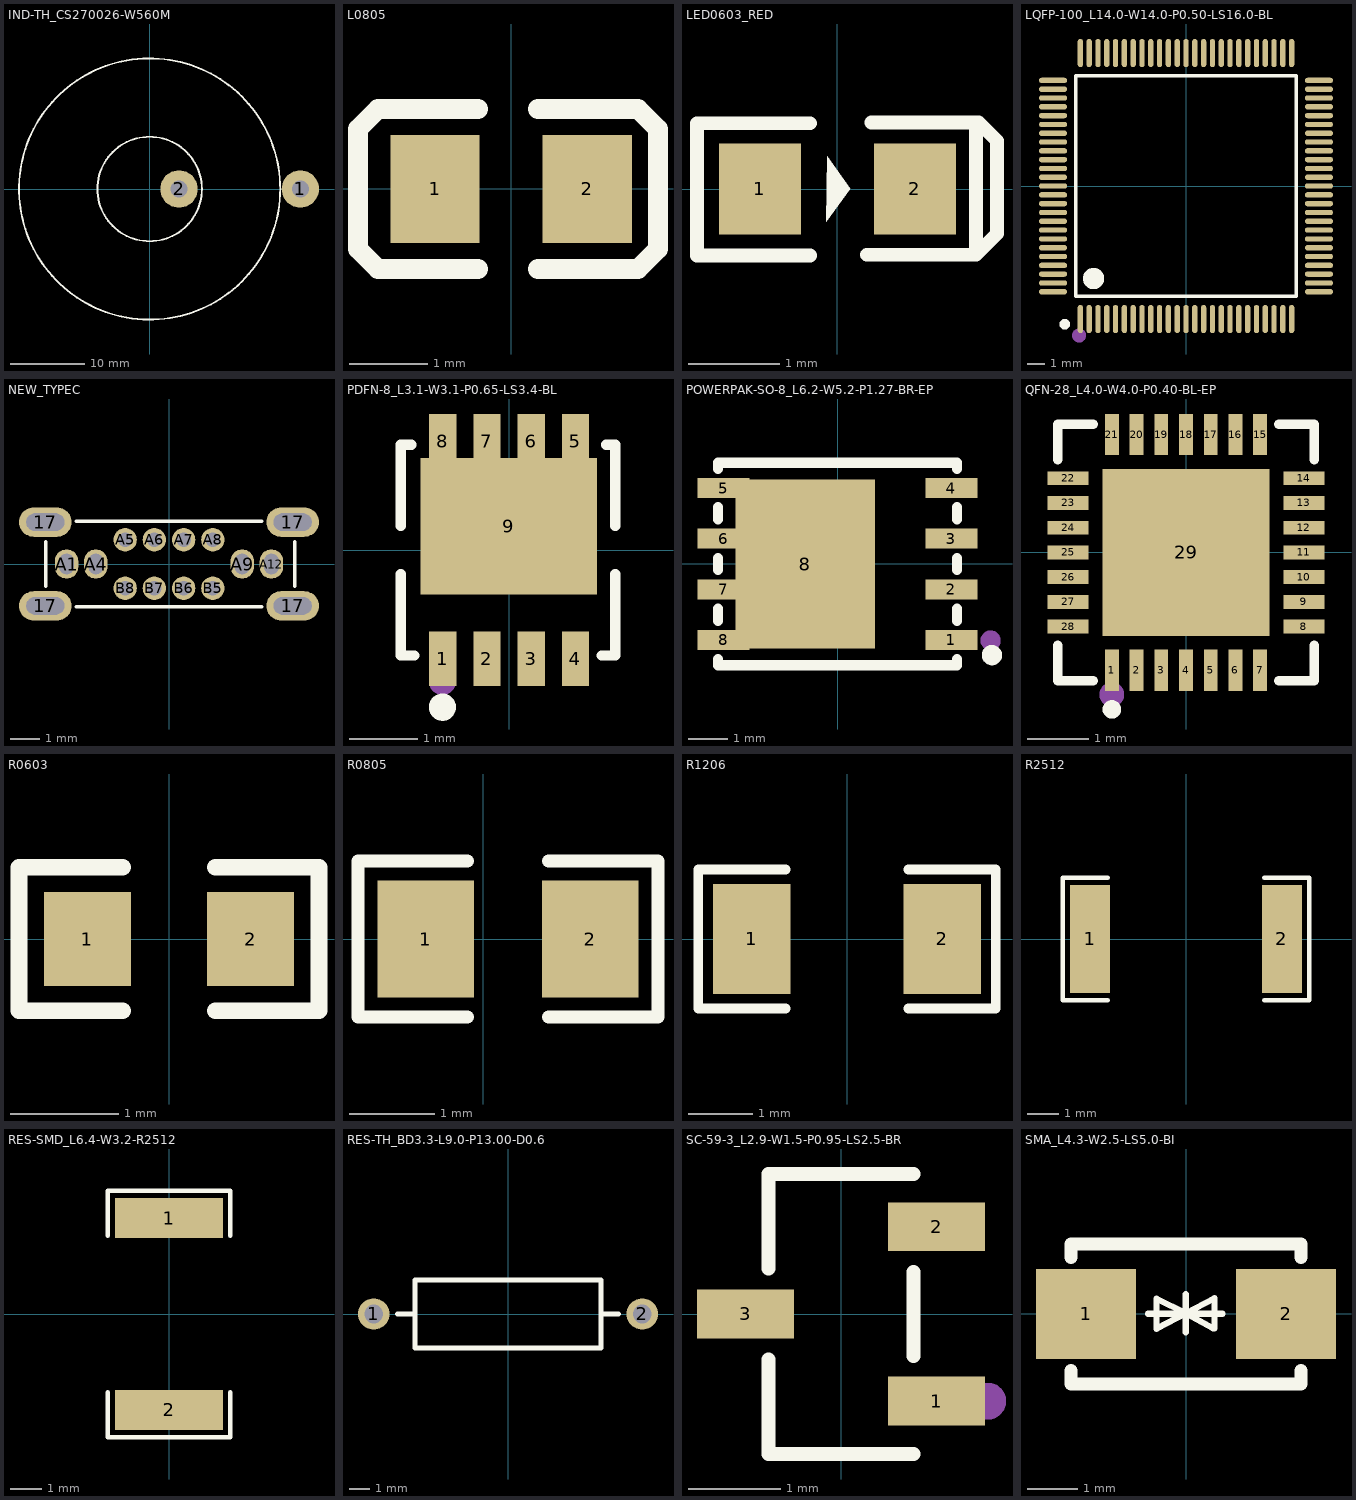
[diagram p0: the footprints below, top view; thin cyan lines are the x and y axes]
# Altium footprint library MISC84402-2.PcbLib: 69 footprints (part 3 of 5)
Each footprint in its own frame and in the unit in brackets; x right, y up, seen from the top. Pads: shape width x height; smd on the part's side, far side on the other; paste and mask are expansions set on the pad; w line width, h text height; cw(c..) or ccw(c..) is an arc to the next point about the centre after c.

## IND-TH_CS270026-W560M [mm]
pads (2):
  round 5 hole 2.3: 1(20.193,0) 2(3.937,0)
Top Overlay:
  circle w0.254: c0,0 r17.5
  circle w0.254: c0,0 r7

## L0805 [mm]
pads (2):
  rect 1.133x1.377 smd: 1(-0.966,0) 2(0.966,0)
Top Overlay:
  lines w0.254: -0.421,-1.016 -1.691,-1.016 -1.945,-0.762 -1.945,-0.635 -1.945,0.762 -1.691,1.016 -1.564,1.016 -0.421,1.016 ; 0.341,-1.016 1.484,-1.016 1.611,-1.016 1.865,-0.762 1.865,0.635 1.865,0.762 1.611,1.016 0.341,1.016
Top Paste:
  region: -0.36,-0.22 -0.36,0.22 -0.745,0.688 -1.433,0.688 -1.533,0.588 -1.533,-0.589 -1.433,-0.689 -0.745,-0.689
  region: 0.36,-0.22 0.36,0.22 0.745,0.688 1.433,0.688 1.533,0.588 1.533,-0.589 1.433,-0.689 0.745,-0.689

## LED0603_RED [mm]
pads (2):
  rect 0.9x1 smd: 1(-0.85,0) 2(0.85,0)
Top Overlay:
  region: -0.11,0.36 -0.12,-0.36 0.14,0
  lines w0.15: -0.3,-0.73 -1.54,-0.73 -1.54,0.72 -0.3,0.72 ; 0.32,-0.72 1.52,-0.72 ; 0.37,0.73 1.52,0.73 ; 1.52,-0.72 1.52,0.73 ; 1.52,-0.72 1.72,-0.52 1.75,-0.49 1.75,0.53 1.55,0.73 1.52,0.73

## LQFP-100_L14.0-W14.0-P0.50-LS16.0-BL [mm]
pads (100):
  oval 0.3x1.6 smd: 1(-6,-7.55) 2(-5.5,-7.55) 3(-5,-7.55) 4(-4.5,-7.55) 5(-4,-7.55) 6(-3.5,-7.55) 7(-3,-7.55) 8(-2.5,-7.55) 9(-2,-7.55) 10(-1.5,-7.55) 11(-1,-7.55) 12(-0.5,-7.55) 13(0,-7.55) 14(0.5,-7.55) 15(1,-7.55) 16(1.5,-7.55) 17(2,-7.55) 18(2.5,-7.55) 19(3,-7.55) 20(3.5,-7.55) 21(4,-7.55) 22(4.5,-7.55) 23(5,-7.55) 24(5.5,-7.55) 25(6,-7.55) 51(6,7.55) 52(5.5,7.55) 53(5,7.55) 54(4.5,7.55) 55(4,7.55) 56(3.5,7.55) 57(3,7.55) 58(2.5,7.55) 59(2,7.55) 60(1.5,7.55) 61(1,7.55) 62(0.5,7.55) 63(0,7.55) 64(-0.5,7.55) 65(-1,7.55) 66(-1.5,7.55) 67(-2,7.55) 68(-2.5,7.55) 69(-3,7.55) 70(-3.5,7.55) 71(-4,7.55) 72(-4.5,7.55) 73(-5,7.55) 74(-5.5,7.55) 75(-6,7.55)
  oval 1.6x0.3 smd: 26(7.55,-6) 27(7.55,-5.5) 28(7.55,-5) 29(7.55,-4.5) 30(7.55,-4) 31(7.55,-3.5) 32(7.55,-3) 33(7.55,-2.5) 34(7.55,-2) 35(7.55,-1.5) 36(7.55,-1) 37(7.55,-0.5) 38(7.55,0) 39(7.55,0.5) 40(7.55,1) 41(7.55,1.5) 42(7.55,2) 43(7.55,2.5) 44(7.55,3) 45(7.55,3.5) 46(7.55,4) 47(7.55,4.5) 48(7.55,5) 49(7.55,5.5) 50(7.55,6) 76(-7.55,6) 77(-7.55,5.5) 78(-7.55,5) 79(-7.55,4.5) 80(-7.55,4) 81(-7.55,3.5) 82(-7.55,3) 83(-7.55,2.5) 84(-7.55,2) 85(-7.55,1.5) 86(-7.55,1) 87(-7.55,0.5) 88(-7.55,0) 89(-7.55,-0.5) 90(-7.55,-1) 91(-7.55,-1.5) 92(-7.55,-2) 93(-7.55,-2.5) 94(-7.55,-3) 95(-7.55,-3.5) 96(-7.55,-4) 97(-7.55,-4.5) 98(-7.55,-5) 99(-7.55,-5.5) 100(-7.55,-6)
Top Overlay:
  lines w0.2: -6.25,-6.25 6.25,-6.25 6.25,6.25 -6.25,6.25 -6.25,-6.25
  lines w0.3: -6.883,-7.696 ccw(c-6.882,-7.846) -6.881,-7.696
  lines w0.6: -5.25,-4.95 ccw(c-5.248,-5.25) -5.245,-4.95
Mechanical 15:
  circle w0.4: c-6.071,-8.484 r0.2

## NEW_TYPEC [mm]
pads (16):
  oval 1.8x1 hole 0.6 slot 1.3 at 0 deg: 17(-4.225,-1.43) 17(-4.225,1.43) 17(4.225,-1.43) 17(4.225,1.43)
  oval 0.8x1 hole 0.5 slot 0.7 at 90 deg: A1(-3.5,0) A4(-2.5,0) A9(2.5,0) A12(3.5,0)
  round 0.8 hole 0.5: A5(-1.5,0.825) A6(-0.5,0.825) A7(0.5,0.825) A8(1.5,0.825) B5(1.5,-0.825) B6(0.5,-0.825) B7(-0.5,-0.825) B8(-1.5,-0.825)
Top Overlay:
  lines w0.127: -4.215,-0.762 -4.215,0.762 ; -3.158,-1.46 3.158,-1.46 ; -3.158,1.461 3.158,1.461 ; 4.294,-0.762 4.294,0.762

## PDFN-8_L3.1-W3.1-P0.65-LS3.4-BL [mm]
pads (9):
  rect 0.4x0.8 smd: 1(-0.975,-1.6) 2(-0.325,-1.6) 3(0.325,-1.6) 4(0.975,-1.6) 5(0.975,1.6) 6(0.325,1.6) 7(-0.325,1.6) 8(-0.975,1.6)
  rect 2.6x2 smd: 9(-0.005,0.35)
Top Overlay:
  circle w0.2: c-0.98,-2.31 r0.1
  lines w0.152: -1.592,-0.354 -1.592,-1.55 -1.396,-1.55 ; -1.592,0.354 -1.592,1.55 -1.434,1.55 ; 1.362,-1.55 1.56,-1.55 1.56,-0.354 ; 1.425,1.55 1.56,1.55 1.56,0.354
Top Paste:
  region: -0.775,1.5 -1.175,1.5 -1.175,2 -0.775,2
  region: 0.775,-2 0.775,-1.2 1.175,-1.2 1.175,-2
  region: 0.125,-2 0.125,-1.2 0.525,-1.2 0.525,-2
  region: -0.525,-2 -0.525,-1.2 -0.125,-1.2 -0.125,-2
  region: -1.175,-2 -1.175,-1.2 -0.775,-1.2 -0.775,-2
  region: -1.31,1.22 1.293,1.22 1.293,-0.649 -1.307,-0.649
  region: -0.125,1.5 -0.525,1.5 -0.525,2 -0.125,2
  region: 0.525,1.5 0.125,1.5 0.125,2 0.525,2
  region: 1.175,1.5 0.775,1.5 0.775,2 1.175,2
Mechanical 15:
  circle w0.2: c-0.98,-1.93 r0.1

## POWERPAK-SO-8_L6.2-W5.2-P1.27-BR-EP [mm]
pads (9):
  rect 1.3x0.5 smd: 1(2.858,-1.905) 2(2.858,-0.635) 3(2.858,0.635) 4(2.858,1.905) 5(-2.858,1.905) 6(-2.858,0.635) 7(-2.858,-0.635) 8(-2.858,-1.905)
  rect 3.5x4.25 smd: 8(-0.813,0)
Top Overlay:
  circle w0.254: c3.873,-2.286 r0.127
  lines w0.254: -3,-2.386 -3,-2.54 3,-2.54 3,-2.386 ; -3,-1.424 -3,-1.116 ; -3,-0.154 -3,0.154 ; -3,1.116 -3,1.424 ; -3,2.386 -3,2.54 3,2.54 3,2.386 ; 3,-1.424 3,-1.116 ; 3,-0.154 3,0.154 ; 3,1.116 3,1.424
Top Paste:
  region: 0.86,1.991 0.86,0.171 -1.94,0.171 -1.94,1.991
  region: -1.94,-1.978 -1.94,-0.158 0.86,-0.158 0.86,-1.978
  region: 2.19,-2.185 2.19,-1.665 3.49,-1.665 3.49,-2.185
  region: 2.19,-0.915 2.19,-0.395 3.49,-0.395 3.49,-0.915
  region: 2.19,0.355 2.19,0.875 3.49,0.875 3.49,0.355
  region: 2.19,1.625 2.19,2.145 3.49,2.145 3.49,1.625
  region: -3.525,-2.185 -3.525,-1.665 -2.225,-1.665 -2.225,-2.185
  region: -3.525,-0.915 -3.525,-0.395 -2.225,-0.395 -2.225,-0.915
  region: -3.525,0.355 -3.525,0.875 -2.225,0.875 -2.225,0.355
  region: -3.525,1.625 -3.525,2.145 -2.225,2.145 -2.225,1.625
Mechanical 15:
  circle w0.254: c3.84,-1.92 r0.127

## QFN-28_L4.0-W4.0-P0.40-BL-EP [mm]
pads (29):
  rect 0.224x0.665 smd: 1(-1.2,-1.907) 2(-0.8,-1.907) 3(-0.4,-1.907) 4(0,-1.907) 5(0.4,-1.907) 6(0.8,-1.907) 7(1.2,-1.907) 15(1.2,1.908) 16(0.8,1.908) 17(0.4,1.908) 18(0,1.908) 19(-0.4,1.908) 20(-0.8,1.908) 21(-1.2,1.908)
  rect 0.665x0.224 smd: 8(1.907,-1.2) 9(1.907,-0.8) 10(1.907,-0.4) 11(1.907,0) 12(1.907,0.4) 13(1.907,0.8) 14(1.907,1.2) 22(-1.907,1.2) 23(-1.907,0.8) 24(-1.907,0.4) 25(-1.907,0) 26(-1.907,-0.4) 27(-1.907,-0.8) 28(-1.907,-1.2)
  rect 2.7x2.7 smd: 29(0,0)
Top Overlay:
  circle w0.15: c-1.2,-2.54 r0.075
  lines w0.152: -2.076,-1.503 -2.076,-2.076 -1.503,-2.076 ; -2.076,1.503 -2.076,2.076 -1.503,2.076 ; 1.503,-2.076 2.076,-2.076 2.076,-1.503 ; 1.503,2.076 2.076,2.076 2.076,1.503
Mechanical 15:
  circle w0.2: c-1.2,-2.3 r0.1

## R0603 [mm]
pads (2):
  rect 0.806x0.864 smd: 1(-0.753,0) 2(0.753,0)
Top Overlay:
  lines w0.152: -0.426,-0.661 -1.385,-0.661 -1.385,0.661 -0.426,0.661 ; 0.426,-0.661 1.385,-0.661 1.385,0.661 0.426,0.661
Top Paste:
  region: -0.355,0.4 -0.355,0.172 -0.735,0.172 -0.735,-0.158 -0.355,-0.158 -0.355,-0.4 -0.405,-0.45 -1.195,-0.45 -1.245,-0.4 -1.245,0.4 -1.195,0.45 -0.405,0.45
  region: 1.195,0.45 0.395,0.45 0.345,0.4 0.345,0.172 0.715,0.172 0.715,-0.158 0.345,-0.158 0.345,-0.4 0.395,-0.45 1.195,-0.45 1.245,-0.4 1.245,0.4

## R0805 [mm]
pads (2):
  rect 1.133x1.377 smd: 1(-0.678,0) 2(1.254,0)
Top Overlay:
  lines w0.152: -0.188,-0.917 -1.473,-0.917 -1.473,0.917 -0.188,0.917 ; 0.764,-0.917 2.049,-0.917 2.049,0.917 0.764,0.917
Top Paste:
  region: -1.412,-0.64 -1.412,0.64 -1.362,0.69 -0.212,0.69 -0.162,0.64 -0.157,0.23 -0.607,0.23 -0.607,-0.22 -0.167,-0.22 -0.162,-0.64 -0.212,-0.69 -1.362,-0.69
  region: 0.738,-0.64 0.738,-0.22 1.183,-0.22 1.183,0.23 0.743,0.23 0.738,0.64 0.788,0.69 1.938,0.69 1.988,0.64 1.988,-0.64 1.938,-0.69 0.788,-0.69

## R1206 [mm]
height 12.5
pads (2):
  rect 1.208x1.701 smd: 1(-1.479,0) 2(1.479,0)
Top Overlay:
  lines w0.152: -0.951,-1.079 -2.311,-1.079 -2.311,1.079 -0.951,1.079 ; 0.951,-1.079 2.311,-1.079 2.311,1.079 0.951,1.079
Top Paste:
  region: 0.875,-0.75 0.875,-0.389 0.975,-0.289 1.186,-0.289 1.286,-0.189 1.286,0.189 1.186,0.289 0.975,0.289 0.875,0.389 0.875,0.75 0.975,0.85 1.983,0.85 2.083,0.75 2.083,-0.75 1.983,-0.85 0.975,-0.85
  region: -0.875,-0.75 -0.875,-0.389 -0.975,-0.289 -1.186,-0.289 -1.286,-0.189 -1.286,0.189 -1.186,0.289 -0.975,0.289 -0.875,0.389 -0.875,0.75 -0.975,0.85 -1.983,0.85 -2.083,0.75 -2.083,-0.75 -1.983,-0.85 -0.975,-0.85

## R2512 [mm]
pads (2):
  rect 1.283x3.456 smd: 1(-3.066,0) 2(3.066,0)
Top Overlay:
  lines w0.152: -2.501,-1.957 -3.936,-1.957 -3.936,1.957 -2.501,1.957 ; 2.501,-1.957 3.936,-1.957 3.936,1.957 2.501,1.957
Top Paste:
  region: -2.425,-1.628 -2.425,-0.688 -2.525,-0.588 -2.761,-0.588 -2.861,-0.488 -2.861,0.488 -2.761,0.588 -2.525,0.588 -2.425,0.688 -2.425,1.628 -2.525,1.728 -3.608,1.728 -3.708,1.628 -3.708,-1.628 -3.608,-1.728 -2.525,-1.728
  region: 2.425,-1.628 2.425,-0.688 2.525,-0.588 2.761,-0.588 2.861,-0.488 2.861,0.488 2.761,0.588 2.525,0.588 2.425,0.688 2.425,1.628 2.525,1.728 3.608,1.728 3.708,1.628 3.708,-1.628 3.608,-1.728 2.525,-1.728

## RES-SMD_L6.4-W3.2-R2512 [mm]
pads (2):
  rect 3.456x1.283 smd: 1(0,3.066) 2(0,-3.066)
Top Overlay:
  lines w0.152: -1.957,-2.501 -1.957,-3.936 1.957,-3.936 1.957,-2.501 ; -1.957,2.501 -1.957,3.936 1.957,3.936 1.957,2.501
Top Paste:
  region: -1.628,2.425 -0.688,2.425 -0.588,2.525 -0.588,2.761 -0.488,2.861 0.488,2.861 0.588,2.761 0.588,2.525 0.688,2.425 1.628,2.425 1.728,2.525 1.728,3.608 1.628,3.708 -1.628,3.708 -1.728,3.608 -1.728,2.525
  region: -1.628,-2.425 -0.688,-2.425 -0.588,-2.525 -0.588,-2.761 -0.488,-2.861 0.488,-2.861 0.588,-2.761 0.588,-2.525 0.688,-2.425 1.628,-2.425 1.728,-2.525 1.728,-3.608 1.628,-3.708 -1.628,-3.708 -1.728,-3.608 -1.728,-2.525

## RES-TH_BD3.3-L9.0-P13.00-D0.6 [mil]
pads (2):
  round 60 hole 36: 1(-255.91,0) 2(255.9,0)
Top Overlay:
  lines w10: -210,0 -180,0 ; 180,0 210,0 ; -177.16,-64.96 177.16,-64.96 177.16,64.96 -177.16,64.96 -177.16,-64.96

## SC-59-3_L2.9-W1.5-P0.95-LS2.5-BR [mm]
pads (3):
  rect 1.058x0.532 smd: 1(1.041,-0.95) 2(1.041,0.95) 3(-1.041,0)
Top Overlay:
  lines w0.152: -0.789,-0.495 -0.789,-1.526 0.789,-1.526 ; -0.789,0.495 -0.789,1.526 0.789,1.526 ; 0.789,-0.455 0.789,0.455
Mechanical 15:
  circle w0.2: c1.6,-0.95 r0.1

## SMA_L4.3-W2.5-LS5.0-BI [mm]
pads (2):
  rect 2x1.8 smd: 1(-2,0) 2(2,0)
Top Overlay:
  lines w0.127: -0.76,0.003 0.73,0.003 ; -0.59,-0.297 -0.59,0.303 -0.002,0.014 ; -0.576,-0.284 -0.004,0.015 ; -0.002,-0.367 -0.002,0.014 ; -0.002,0.395 -0.002,0.014 ; 0.54,-0.287 -0.002,0.014 ; 0.57,-0.287 0.57,0.313 -0.002,0.014
  lines w0.254: -2.3,-1.131 -2.3,-1.4 2.3,-1.4 2.3,-1.131 ; -2.3,1.131 -2.3,1.4 2.3,1.4 2.3,1.131